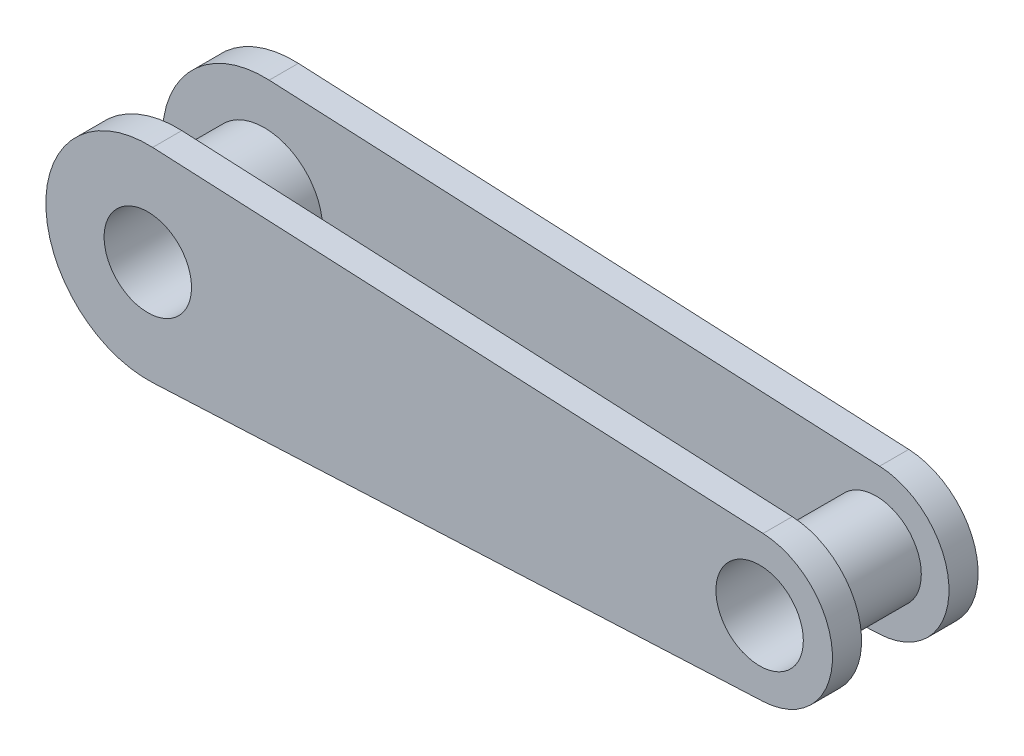
SolidWorks part; units mm, degrees
ref_plane "Front Plane" through (0, 0, 0) normal (0, 0, 1) x (1, 0, 0)
ref_plane "Top Plane" through (0, 0, 0) normal (0, 1, 0) x (1, 0, 0)
ref_plane "Right Plane" through (0, 0, 0) normal (1, 0, 0) x (0, 0, -1)
other "Configuration Table"
sketch "Sketch1" plane through (0, 0, 0) normal (0, 0, 1) x (1, 0, 0)
  line L0 (1.6667, 34.9603) -> (211.1905, 24.9716)
  line L1 (1.6667, -34.9603) -> (211.1905, -24.9716)
  line L2 (0, 0) -> (185, 0) construction
  arc A0 (1.6667, 34.9603) -> (1.6667, -34.9603) centre (0, 0) ccw
  arc A1 (211.1905, -24.9716) -> (211.1905, 24.9716) centre (210, 0) ccw
  dimension "D1" = 210
  dimension "60" = 70
  dimension "D3" = 50
extrude "Boss-Extrude1" add sketch "Sketch1" along normal blind 10
sketch "Sketch3" plane through (0, 0, 0) normal (0, 0, -1) x (-1, 0, 0)
  circle A0 centre (0, 0) radius 20
  circle A1 centre (0, 0) radius 15
  circle A2 centre (-210, 0) radius 15
  circle A3 centre (-210, 0) radius 15.5
  dimension "D1" = 30
  dimension "D2" = 31
  dimension "D3" = 30
  dimension "D4" = 40
extrude "Boss-Extrude2" add sketch "Sketch3" along normal blind 30
sketch "Sketch5" plane through (0, 0, -30) normal (0, 0, -1) x (-1, 0, 0)
  circle A0 centre (0, 0) radius 15 construction
  circle A1 centre (-210, 0) radius 15.5
  circle A2 centre (-210, 0) radius 15.5
  circle A3 centre (0, 0) radius 20
  circle A4 centre (0, 0) radius 20
  circle A5 centre (0, 0) radius 15
  circle A6 centre (-210, 0) radius 15 construction
  circle A7 centre (-210, 0) radius 15
  dimension "D1" = 0
  dimension "D2" = 0
extrude "Cut-Extrude1" cut sketch "Sketch5" against normal blind 106 contours A7 | A5
sketch "Sketch6" plane through (0, 0, 0) normal (0, 0, -1) x (-1, 0, 0)
  line L2 (-1.6667, 34.9603) -> (-211.1905, 24.9716)
  line L3 (-211.1905, -24.9716) -> (-1.6667, -34.9603)
  line L4 (-1.6667, 34.9603) -> (-211.1905, 24.9716)
  line L5 (-211.1905, -24.9716) -> (-1.6667, -34.9603)
  arc A2 (-1.6667, -34.9603) -> (-1.6667, 34.9603) centre (0, 0) ccw
  arc A3 (-211.1905, 24.9716) -> (-211.1905, -24.9716) centre (-210, 0) ccw
  arc A4 (-1.6667, -34.9603) -> (-1.6667, 34.9603) centre (0, 0) ccw
  arc A5 (-211.1905, 24.9716) -> (-211.1905, -24.9716) centre (-210, 0) ccw
  dimension "D1" = 0
extrude "Boss-Extrude3" add sketch "Sketch6" along normal blind 10 from offset 30 separate body
sketch "Sketch7" plane through (0, 0, -30) normal (0, 0, 1) x (1, 0, 0)
  line L2 (1.6667, -34.9603) -> (211.1905, -24.9716)
  line L3 (211.1905, 24.9716) -> (1.6667, 34.9603)
  line L4 (1.6667, -34.9603) -> (211.1905, -24.9716)
  line L5 (211.1905, 24.9716) -> (1.6667, 34.9603)
  circle A0 centre (210, 0) radius 15 construction
  circle A1 centre (0, 0) radius 15 construction
  arc A2 (1.6667, 34.9603) -> (1.6667, -34.9603) centre (0, 0) ccw
  arc A3 (211.1905, -24.9716) -> (211.1905, 24.9716) centre (210, 0) ccw
  arc A4 (1.6667, 34.9603) -> (1.6667, -34.9603) centre (0, 0) ccw
  arc A5 (211.1905, -24.9716) -> (211.1905, 24.9716) centre (210, 0) ccw
  circle A6 centre (210, 0) radius 15
  circle A7 centre (0, 0) radius 15
  dimension "D1" = 0
extrude "Cut-Extrude2" cut sketch "Sketch7" against normal blind 110 contours A7 | A6
